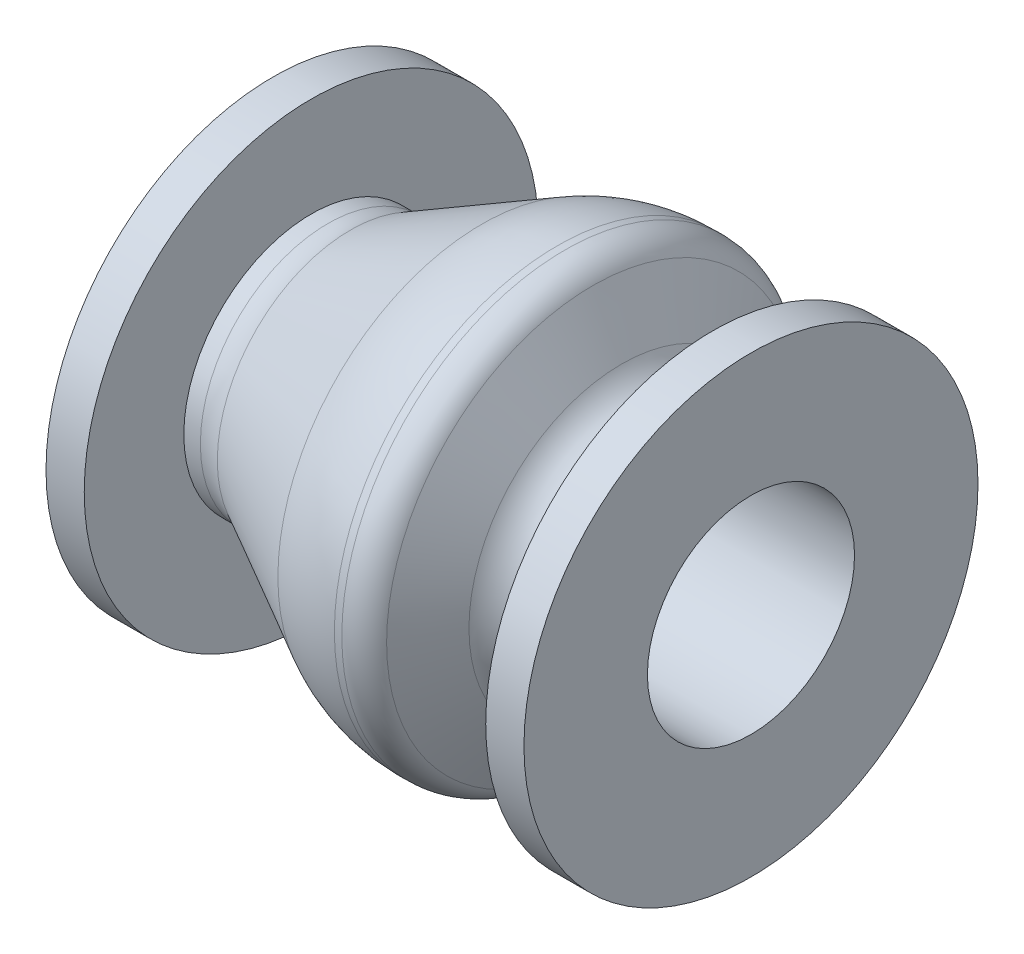
SolidWorks part; units mm, degrees
material "铸造碳钢"
ref_plane "Front Plane" through (0, 0, 0) normal (0, 0, 1) x (1, 0, 0)
ref_plane "Top Plane" through (0, 0, 0) normal (0, 1, 0) x (1, 0, 0)
ref_plane "Right Plane" through (0, 0, 0) normal (1, 0, 0) x (0, 0, -1)
sketch "Sketch1" plane through (0, 0, 0) normal (0, 0, 1) x (1, 0, 0)
  line L0 (0, 65) -> (0, 142.5)
  line L1 (0, 142.5) -> (24, 142.5)
  line L2 (24, 142.5) -> (24, 80)
  line L3 (24, 80) -> (34.3984, 80)
  line L4 (48.6214, 83.5859) -> (130.9805, 127.933)
  line L5 (178.3905, 139.8859) -> (183.0579, 139.8859)
  line L6 (200.6673, 129.3679) -> (218.7548, 95.777)
  line L7 (245.1689, 80) -> (276, 80)
  line L8 (276, 80) -> (276, 142.5)
  line L9 (276, 142.5) -> (300, 142.5)
  line L10 (300, 142.5) -> (300, 65)
  line L11 (300, 65) -> (0, 65)
  line L12 (0, 0) -> (45.6274, 0) construction
  arc A0 (218.7548, 95.777) -> (245.1689, 80) centre (245.1689, 110) ccw
  arc A1 (34.3984, 80) -> (48.6214, 83.5859) centre (34.3984, 110) ccw
  arc A2 (130.9805, 127.933) -> (178.3905, 139.8859) centre (178.3905, 39.8859) cw
  arc A3 (183.0579, 139.8859) -> (200.6673, 129.3679) centre (183.0579, 119.8859) cw
  dimension "D8" = 30
  dimension "D9" = 100
  dimension "D10" = 20
  dimension "D1" = 142.5
  dimension "D2" = 142.5
  dimension "D3" = 24
  dimension "D4" = 24
  dimension "D5" = 65
  dimension "D6" = 80
  dimension "D7" = 80
  dimension "D11" = 300
revolve "Revolve1" add sketch "Sketch1" angle 360 about L12
